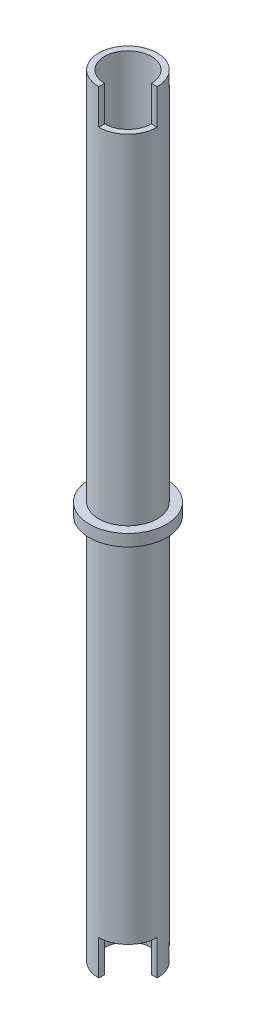
from build123d import *

# Parameters (mm, degrees)
CUT_EXTRUDE1_REACH = 663.648
SKETCH2_R          = 20
CUT_EXTRUDE2_DEPTH = 30
CUT_EXTRUDE3_DEPTH = 30


with BuildPart() as part:
    # Sketch1 → Revolve1 (revolve)
    with BuildSketch(Plane.XY, mode=Mode.PRIVATE) as revolve1_sk:
        Polygon((0, 0), (25, 0), (25, 330), (33, 330), (33, 340), (25, 340), (25, 585.119663834), (25, 619.032357738), (25, 660), (0, 660), align=None)
    revolve(revolve1_sk.sketch.rotate(Axis((0, 660, 0), (0, -1, 0)), 180), axis=Axis((0, 660, 0), (0, -1, 0)))

    # Sketch2 → Cut-Extrude1 (cut, up to next)
    with BuildSketch(Plane(origin=(0, 660, 0), x_dir=(1, 0, 0), z_dir=(0, 1, 0)), mode=Mode.PRIVATE) as cut_extrude1_sk1:
        with Locations(Location((0, 0, 0), (0, 0, 180))):
            Circle(SKETCH2_R)
    cut_extrude1_tool1 = extrude(cut_extrude1_sk1.sketch, amount=-CUT_EXTRUDE1_REACH, mode=Mode.PRIVATE) & part.part
    add(cut_extrude1_tool1.solids().sort_by_distance((0, 660, 0))[0], mode=Mode.SUBTRACT)

    # Sketch3 → Cut-Extrude2 (cut)
    with BuildSketch(Plane(origin=(0, 660, 0), x_dir=(1, 0, 0), z_dir=(0, 1, 0))):
        with BuildLine():
            Line((0, -43.201505936), (0, 0))
            Line((0, 0), (43.201505936, 0))
            ThreePointArc((43.201505936, 0), (30.548077804, -30.548077804), (0, -43.201505936))
        make_face()
    extrude(amount=-CUT_EXTRUDE2_DEPTH, mode=Mode.SUBTRACT)

    # Sketch4 → Cut-Extrude3 (cut)
    with BuildSketch(Plane.XZ):
        with BuildLine():
            Line((51.068202024, 0), (0, 0))
            Line((0, 0), (0, 51.068202024))
            ThreePointArc((0, 51.068202024), (36.110671954, 36.110671954), (51.068202024, 0))
        make_face()
    extrude(amount=-CUT_EXTRUDE3_DEPTH, mode=Mode.SUBTRACT)


solid = part.part
